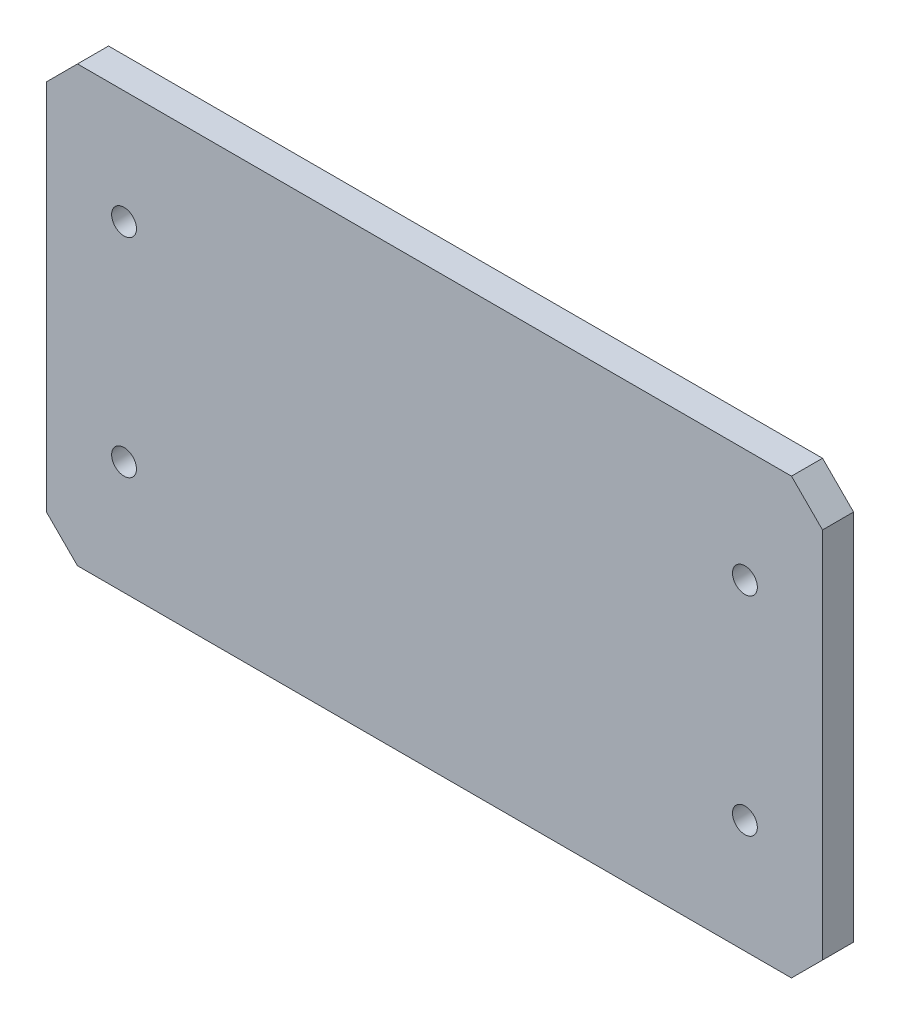
SolidWorks part; units mm, degrees
ref_plane "Front Plane" through (0, 0, 0) normal (0, 0, 1) x (1, 0, 0)
ref_plane "Top Plane" through (0, 0, 0) normal (0, 1, 0) x (1, 0, 0)
ref_plane "Right Plane" through (0, 0, 0) normal (1, 0, 0) x (0, 0, -1)
sketch "Sketch1" plane through (0, 0, 0) normal (0, 0, 1) x (1, 0, 0)
  line L0 (-115, 70) -> (-125, 60)
  line L1 (115, -70) -> (-115, -70)
  line L2 (125, -60) -> (125, 60)
  line L3 (115, 70) -> (-115, 70)
  line L4 (-125, -60) -> (-125, 60)
  line L5 (125, -70) -> (-125, 70) construction
  line L6 (125, 70) -> (-125, -70) construction
  line L7 (-115, -70) -> (-125, -60)
  line L8 (115, -70) -> (125, -60)
  line L9 (125, 60) -> (115, 70)
  point P0 (0, 0)
  dimension "D1" = 250
  dimension "D2" = 140
extrude "Boss-Extrude1" add sketch "Sketch1" along normal blind 10
sketch "Sketch6" plane through (0, 0, 0) normal (0, 0, -1) x (-1, 0, 0)
  line L0 (75, -55) -> (75, 55) construction
  line L1 (0, 0) -> (79.1, 0) construction
  line L2 (0, 76.0031) -> (0, 0) construction
  line L3 (-125, -60) -> (-125, 60) construction
  circle A0 centre (79.1, 0) radius 4
  circle A1 centre (-79.1, 0) radius 4
  dimension "D1" = 8
  dimension "D2" = 8
  dimension "D3" = 49.9
extrude "Cut-Extrude3" cut sketch "Sketch6" against normal blind 5
sketch "Sketch7" plane through (0, 0, 5) normal (0, 0, -1) x (-1, 0, 0)
  circle A1 centre (79.1, 0) radius 4
  circle A2 centre (79.1, 0) radius 4
  dimension "D1" = 0
extrude "Boss-Extrude3" add sketch "Sketch7" along normal up to surface (5 mm away) up to face at (-83.1, 0, 0)
sketch "Sketch8" plane through (0, 0, 0) normal (0, 0, -1) x (-1, 0, 0)
  line L0 (0, 0) -> (0, -64.1) construction
  line L1 (50, -64.1) -> (-50, -64.1) construction
  line L2 (115, -70) -> (-115, -70) construction
  circle A0 centre (-50, -64.1) radius 4
  circle A1 centre (50, -64.1) radius 4
  dimension "D1" = 8
  dimension "D2" = 50
  dimension "D3" = 5.9
extrude "Cut-Extrude4" cut sketch "Sketch8" against normal blind 5
sketch "Sketch11" plane through (0, 0, 10) normal (0, 0, 1) x (1, 0, 0)
  line L0 (0, 96.5714) -> (0, 0) construction
  line L1 (0, 0) -> (189.1584, 0) construction
  circle A1 centre (100, 33.5) radius 4
  circle A2 centre (-100, 33.5) radius 4
  circle A3 centre (-100, -33.5) radius 4
  circle A4 centre (100, -33.5) radius 4
  dimension "D1" = 8
extrude "Cut-Extrude5" cut sketch "Sketch11" against normal up to surface (10 mm away) up to face at (46, -64.1, 0)
